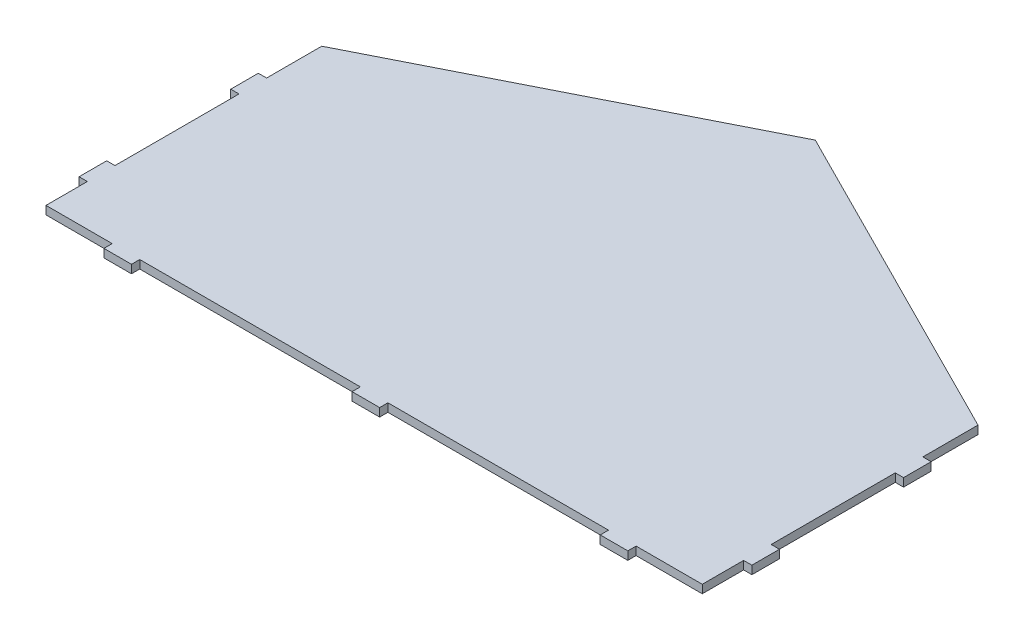
from build123d import *

# Parameters (mm, degrees)
BOSS_EXTRUDE1_DEPTH = 3
SKETCH3_W           = 3
SKETCH3_H           = 10
SKETCH3_W_2         = 10
SKETCH3_H_2         = 3
BOSS_EXTRUDE2_DEPTH = 3


with BuildPart() as part:
    # Sketch1 → Boss-Extrude1 (new body)
    with BuildSketch(Plane(origin=(0, 0, 0), x_dir=(1, 0, 0), z_dir=(0, 1, 0))):
        Polygon((-119, 50), (0, 110), (119, 50), (119, -50), (-119, -50), align=None)
    extrude(amount=BOSS_EXTRUDE1_DEPTH)

    # Sketch3 → Boss-Extrude2 (add)
    with BuildSketch(Plane(origin=(0, 3, 0), x_dir=(1, 0, 0), z_dir=(0, 1, 0))):
        with Locations((120.5, 25)):
            Rectangle(SKETCH3_W, SKETCH3_H)
        with Locations((120.5, -30)):
            Rectangle(SKETCH3_W, SKETCH3_H)
        with Locations((-120.5, -30)):
            Rectangle(SKETCH3_W, SKETCH3_H)
        with Locations((-120.5, 25)):
            Rectangle(SKETCH3_W, SKETCH3_H)
        with Locations((-90, -51.5)):
            Rectangle(SKETCH3_W_2, SKETCH3_H_2)
        with Locations((90, -51.5)):
            Rectangle(SKETCH3_W_2, SKETCH3_H_2)
        with Locations((0, -51.5)):
            Rectangle(SKETCH3_W_2, SKETCH3_H_2)
    extrude(amount=-BOSS_EXTRUDE2_DEPTH)


solid = part.part
